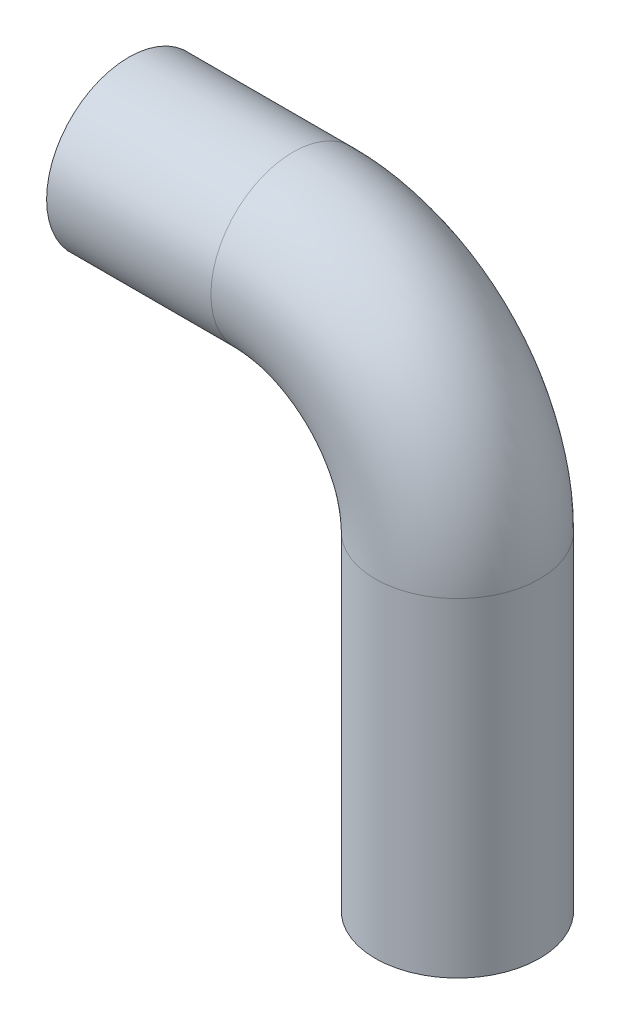
SolidWorks part; units mm, degrees
ref_plane "Front Plane" through (0, 0, 0) normal (0, 0, 1) x (1, 0, 0)
ref_plane "Top Plane" through (0, 0, 0) normal (0, 1, 0) x (1, 0, 0)
ref_plane "Right Plane" through (0, 0, 0) normal (1, 0, 0) x (0, 0, -1)
sketch "Sketch1" plane through (0, 0, 0) normal (0, 0, 1) x (1, 0, 0)
  line L0 (0, 0) -> (10, 0)
  line L1 (20, -10) -> (20, -30)
  arc A0 (10, 0) -> (20, -10) centre (10, -10) cw
  dimension "D1" = 10
sketch "Sketch2" plane through (0, 0, 0) normal (1, 0, 0) x (0, 0, -1)
  circle A0 centre (0, 0) radius 5
  circle A1 centre (0, 0) radius 4
sweep "Sweep1" add profiles "Sketch2" path "Sketch1"
